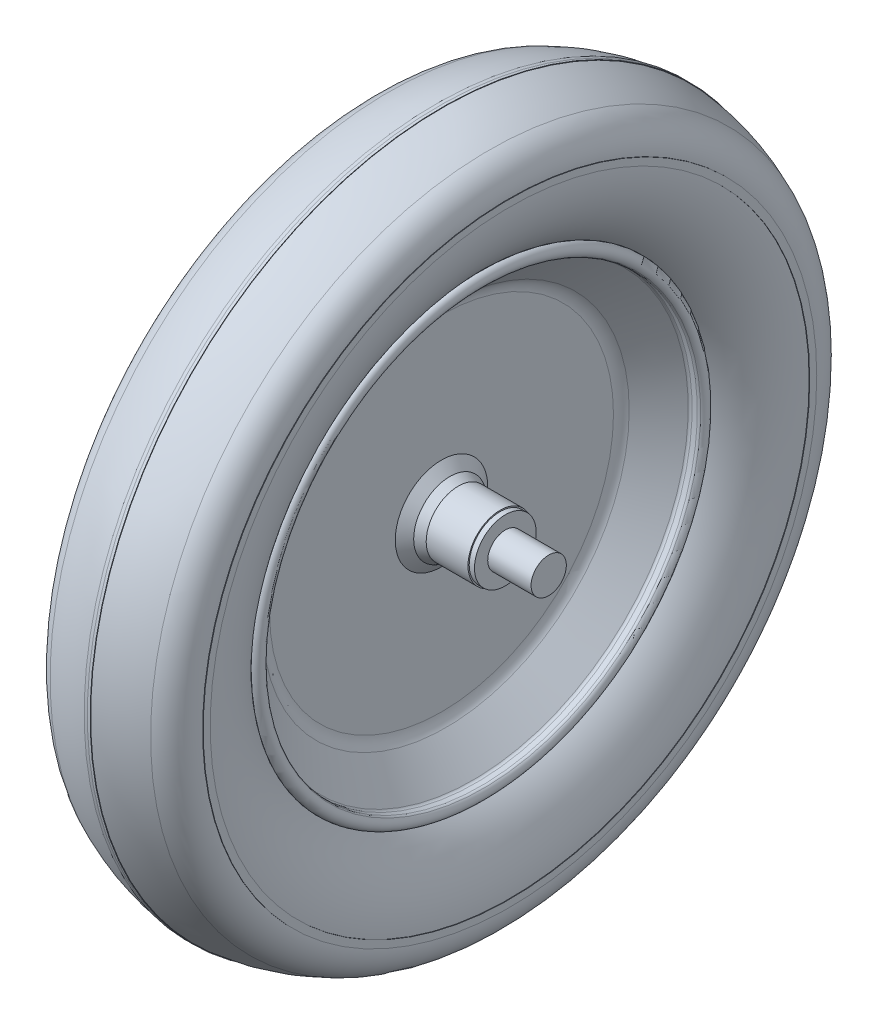
SolidWorks part; units mm, degrees
ref_plane "Front Plane" through (0, 0, 0) normal (0, 0, 1) x (1, 0, 0)
ref_plane "Top Plane" through (0, 0, 0) normal (0, 1, 0) x (1, 0, 0)
ref_plane "Right Plane" through (0, 0, 0) normal (1, 0, 0) x (0, 0, -1)
sketch "Sketch1" plane through (0, 0, 0) normal (0, 0, 1) x (1, 0, 0)
  line L0 (-118.9548, -29.7396) -> (119.5947, -29.7396) construction
  line L1 (41.3877, -19.7396) -> (42.8877, -19.7396)
  line L2 (42.8877, -19.7396) -> (42.8877, -12.2396)
  line L3 (39.8877, -11.5396) -> (16.1877, -11.5396)
  line L4 (16.1877, -11.5396) -> (11.3877, -9.2396)
  line L5 (11.3877, -9.2396) -> (6.6877, -3.4896)
  line L7 (9.1043, 74.3129) -> (24.5777, 92.3141)
  line L8 (26.0944, 93.0104) -> (29.0486, 93.0104)
  line L9 (39.8877, -11.5396) -> (39.8877, -12.2396)
  line L10 (39.8877, -12.2396) -> (42.8877, -12.2396)
  line L11 (6.6877, -3.4896) -> (6.6877, 67.7943)
  line L12 (5.9377, -29.7396) -> (5.9377, 34.5388) construction
  line L13 (38.3877, -13.7396) -> (38.3877, -19.7396)
  line L14 (38.3877, -13.0396) -> (38.3877, -13.7396)
  line L15 (38.3877, -13.0396) -> (15.8469, -13.0396)
  line L16 (15.8469, -13.0396) -> (10.438, -10.4479)
  line L17 (10.438, -10.4479) -> (5.1877, -4.0247)
  line L18 (5.1877, -4.0247) -> (5.1877, 68.3504)
  line L20 (7.6043, 74.8689) -> (23.4402, 93.2918)
  line L21 (26.0944, 94.5104) -> (29.0486, 94.5104)
  line L22 (38.3877, -19.7396) -> (41.3877, -19.7396)
  line L23 (28.6762, 100.2604) -> (28.4732, 98.7604)
  line L24 (-52.8767, 100.2604) -> (98.7925, 100.2604) construction
  arc A0 (30.4002, 93.5362) -> (28.6762, 100.2604) centre (27.7402, 96.4373) ccw
  arc A1 (30.4002, 93.5362) -> (29.0486, 93.0104) centre (29.0486, 95.0104) cw
  arc A2 (24.5777, 92.3141) -> (26.0944, 93.0104) centre (26.0944, 91.0104) cw
  arc A3 (5.1877, 68.3504) -> (7.6043, 74.8689) centre (15.1877, 68.3504) cw
  arc A4 (6.6877, 67.7943) -> (9.1043, 74.3129) centre (16.6877, 67.7943) cw
  arc A7 (23.4402, 93.2918) -> (26.0944, 94.5104) centre (26.0944, 91.0104) cw
  arc A8 (29.3865, 94.6418) -> (29.0486, 94.5104) centre (29.0486, 95.0104) cw
  arc A9 (29.3865, 94.6418) -> (28.4732, 98.7604) centre (27.7402, 96.4373) ccw
  dimension "D7" = 2
  dimension "D13" = 10
  dimension "D1" = 7.5
  dimension "D2" = 8.2
  dimension "D3" = 3
  dimension "D4" = 26.7
  dimension "D5" = 31.5
  dimension "D6" = 36.2
  dimension "D8" = 1.5
  dimension "D9" = 41
  dimension "D10" = 20
  dimension "D11" = 52.5
  dimension "D12" = 130
revolve "Revolve1" add sketch "Sketch1" angle 360 about L0
sketch "Sketch2" plane through (0, 0, 0) normal (0, 0, 1) x (1, 0, 0)
  line L0 (28.5979, 100.2913) -> (28.3949, 98.7913)
  line L1 (28.3949, 98.7913) -> (28.3949, 95.3135)
  line L2 (42.2203, 145.141) -> (42.2096, 139.8046)
  line L3 (27.8949, 94.8135) -> (27.7357, 94.8135)
  line L4 (25.7357, 96.8135) -> (25.7357, 100.8543)
  line L5 (45.1979, 140.2913) -> (45.4979, 140.2913)
  line L6 (45.1979, 144.2913) -> (45.4979, 144.2913)
  line L7 (45.4979, 140.2913) -> (45.4979, 144.2913)
  line L8 (3.4979, 169.7913) -> (3.4979, 166.7848)
  line L9 (51.3015, -29.7396) -> (-34.2178, -29.7396) construction
  arc A0 (28.5979, 100.2913) -> (45.1979, 140.2913) centre (-7.4638, 138.7014) ccw
  arc A1 (45.1979, 144.2913) -> (33.6979, 162.2913) centre (26.7874, 145.2027) ccw
  arc A2 (3.4979, 169.7913) -> (33.6979, 162.2913) centre (-2.1525, 82.4867) cw
  arc A3 (3.4979, 166.7848) -> (32.5223, 159.5306) centre (-2.1525, 82.4867) cw
  arc A4 (42.2203, 145.141) -> (32.5223, 159.5306) centre (26.7874, 145.2027) ccw
  arc A5 (26.3736, 102.3188) -> (42.2096, 139.8046) centre (-7.4638, 138.7014) ccw
  arc A6 (27.7357, 94.8135) -> (25.7357, 96.8135) centre (27.7357, 96.8135) cw
  arc A7 (26.3736, 102.3188) -> (25.7357, 100.8543) centre (27.7357, 100.8543) ccw
  arc A8 (28.3949, 95.3135) -> (27.8949, 94.8135) centre (27.8949, 95.3135) cw
  point P6 (41.1979, 118.5068)
  point P10 (33.6979, 162.2913)
  dimension "D3" = 2
  dimension "D4" = 0.5
  dimension "D1" = 4
  dimension "D2" = 0.3
revolve "Revolve2" add sketch "Sketch2" angle 360 about L9
mirror "Mirror8" about plane through (5.1877, -4.0247, 0) normal (1, 0, 0) of bodies 106 107
sketch "Sketch3" plane through (-32.5123, 0, 0) normal (-1, 0, 0) x (0, 0, 1)
  circle A0 centre (0, -29.7396) radius 10
extrude "Boss-Extrude1" add sketch "Sketch3" along normal blind 25 and the other way blind 100
